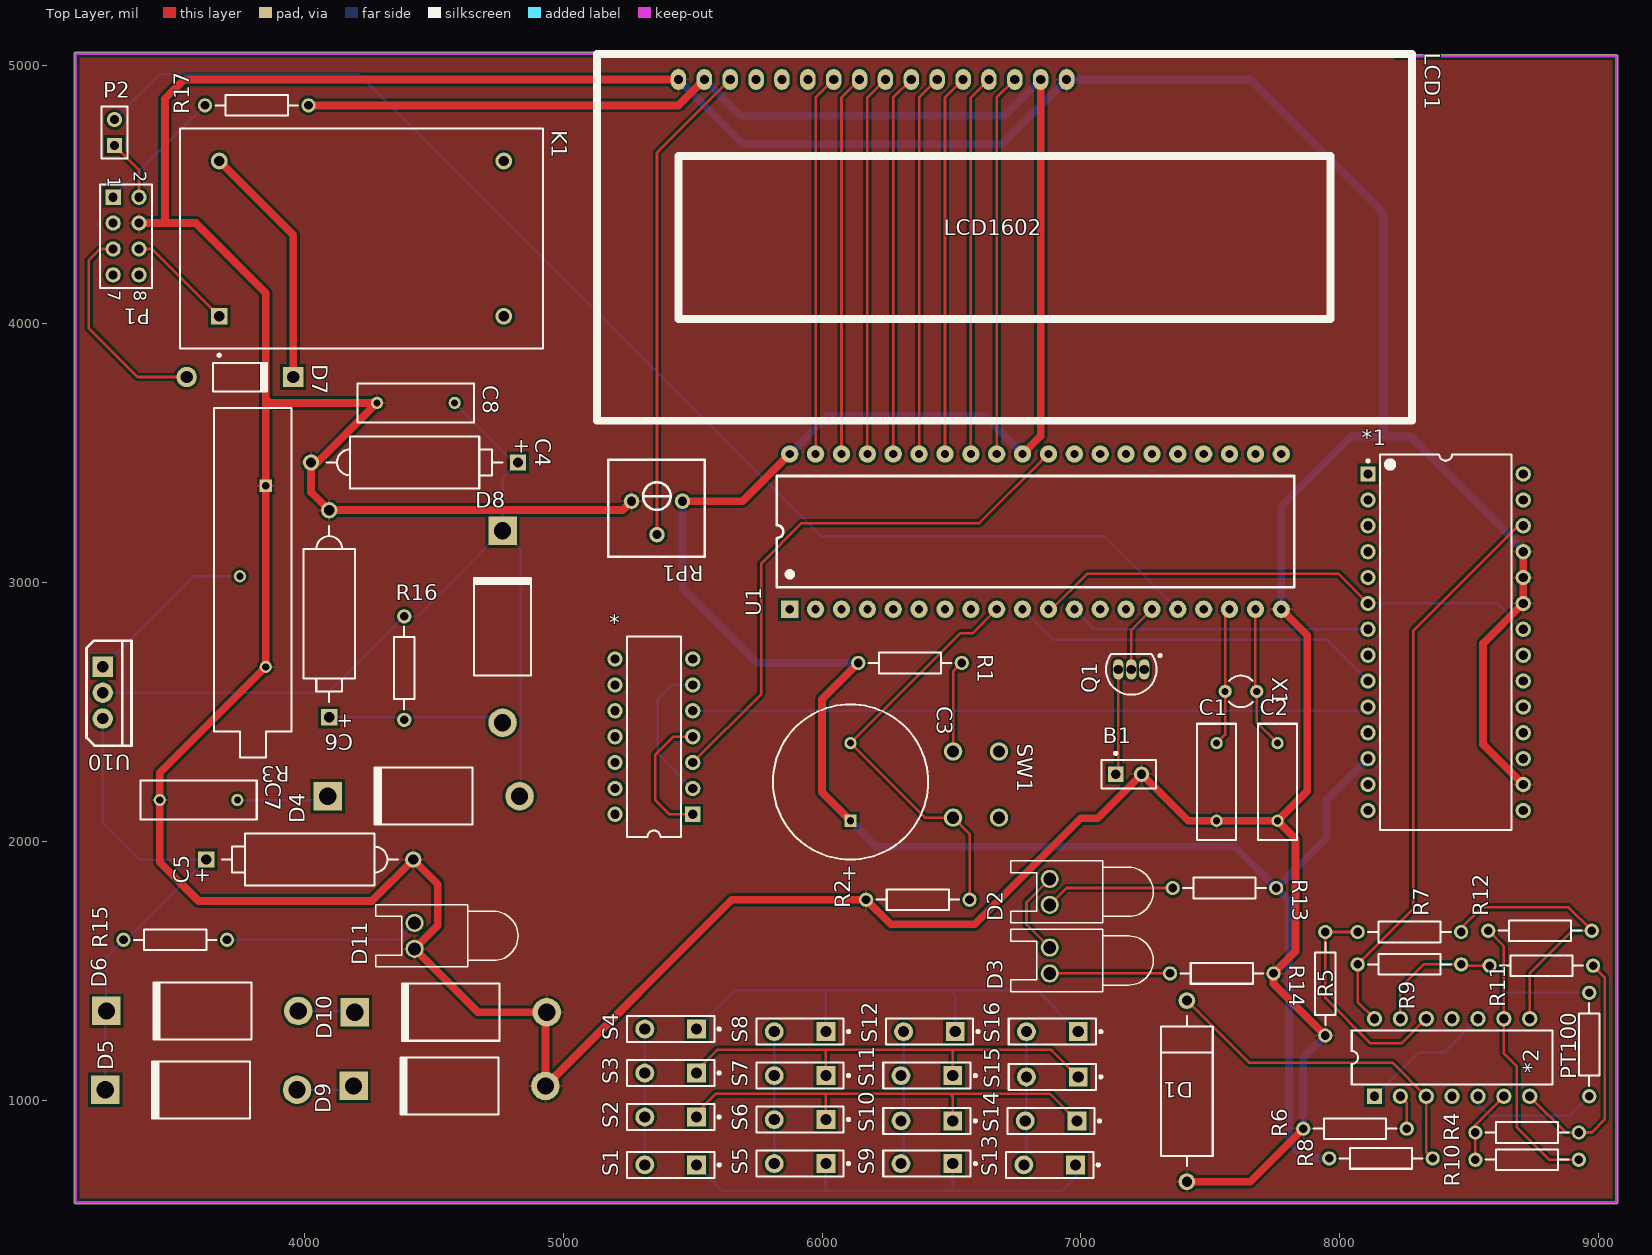
[diagram p0: Top Layer view]
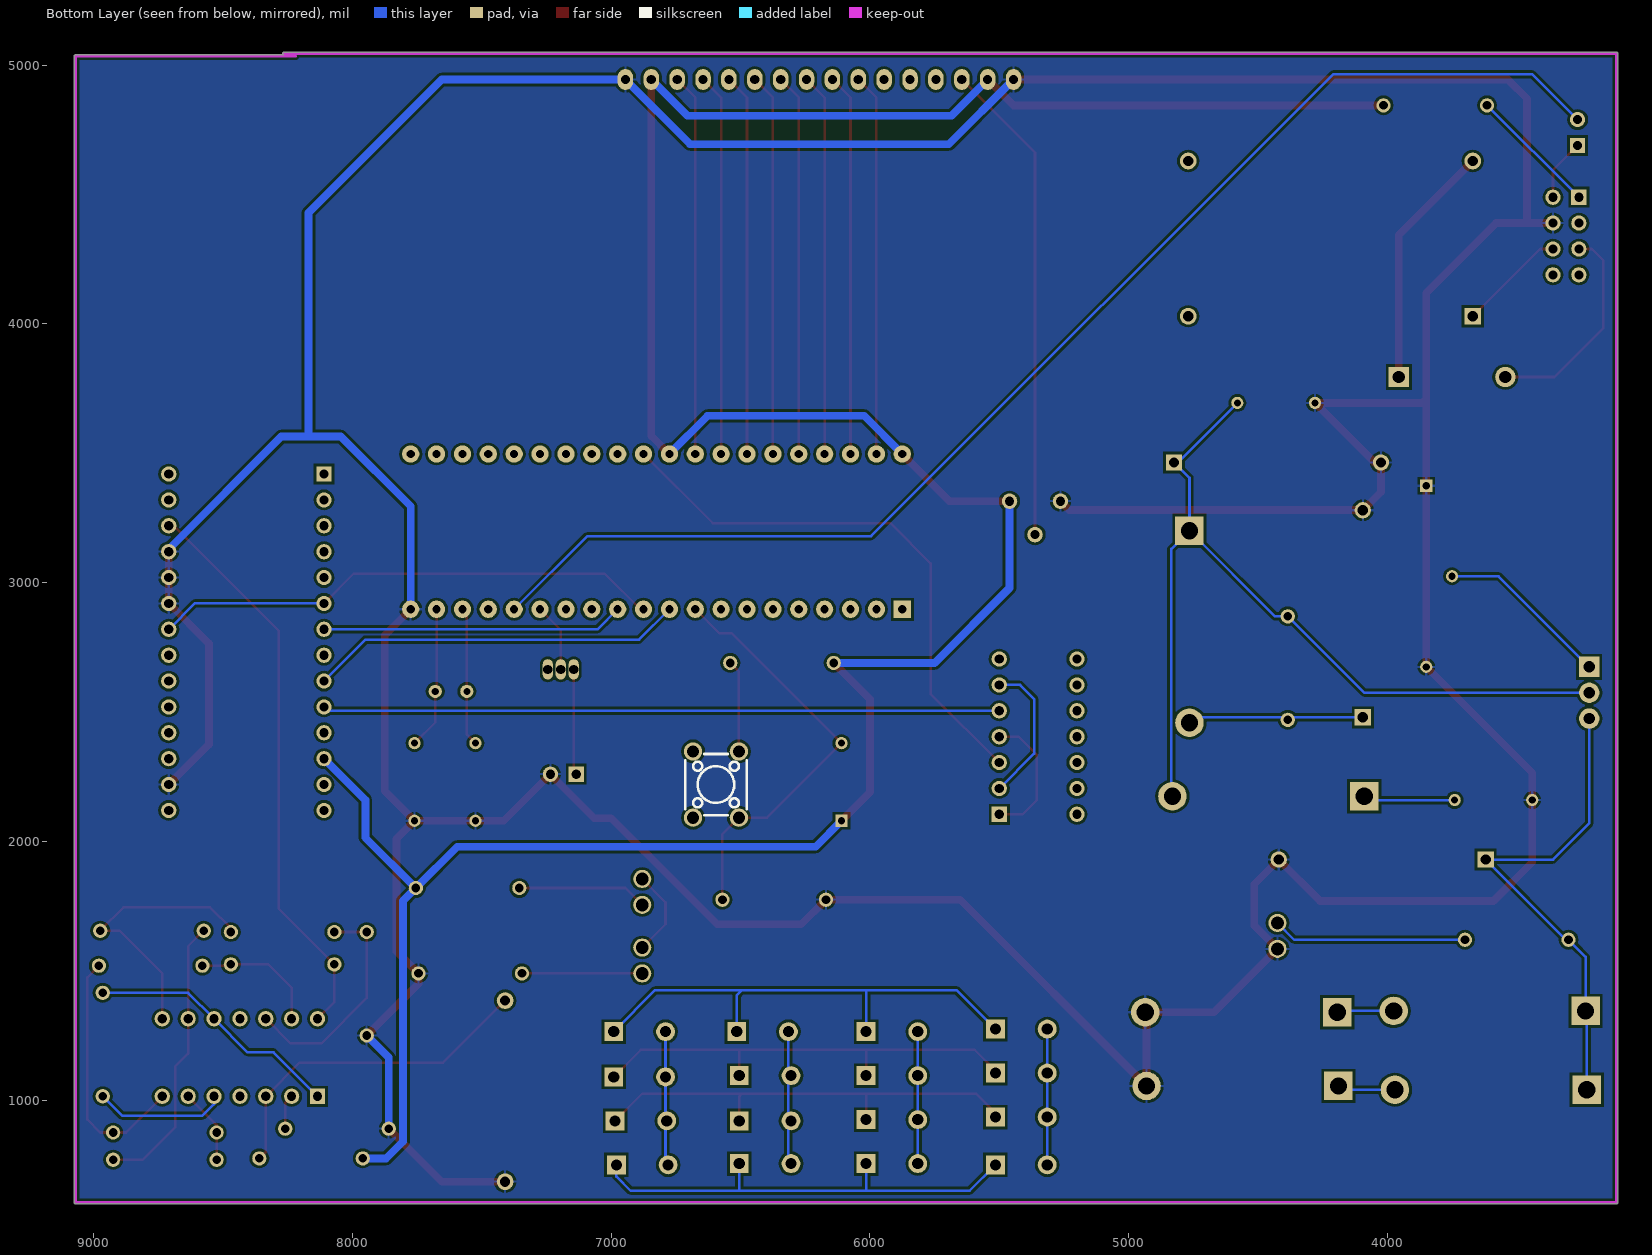
[diagram p1: Bottom Layer view, seen from below]
# Altium PCB MISC80626.PcbDoc
Units mil, origin at the board's own origin, x right, y up, seen from the top; angles counter-clockwise.
Board outline 5965.03 x 4450.03 mil, 2 copper layers (Top Layer, Bottom Layer); 67 components, 63 nets, 250 pads, 0 vias.

## Layer stack, top to bottom (the 12.6 mil dielectric is the usual default, probably not edited)
Top Solder: solder mask 0.4, Solder Resist, Dk 3.5
Top Layer: signal copper 1.4
Dielectric 1: dielectric 12.6, FR-4, Dk 4.8
Bottom Layer: signal copper 1.4
Bottom Solder: solder mask 0.4, Solder Resist, Dk 3.5

## Board outline
3109.99,605 ccw(c3115,605) 3115,599.99 9070,599.99 ccw(c9070,605) 9075.01,605 9075.01,5035 ccw(c9070,5035) 9070,5040.02 8265.55,5040.02 ccw(c8265,5045) 8270.01,5045 ccw(c8265,5045) 8265,5050.02 3115,5050.02 ccw(c3115,5045) 3109.99,5045

## Design rules (kind name [scope] priority, off if disabled: settings)
Clearance [All] p1: gap=10 ignorepadtopadclearanceinfootprint=FALSE except(0: Arc-Hole Track-Hole SMDPad-Hole THPad-Hole Via-Hole Fill-Hole Poly-Hole Region-Hole Text-Hole)
MinimumSolderMaskSliver [All] p1: minsoldermaskwidth=0
PolygonConnect [All] p1: connectstyle=Relief reliefconductorwidth=10 reliefentries=4 polygonreliefangle="90 Angle" airgapwidth=10
RoutingVias [All] p1: holewidth=28 width=50 viastyle="Through Hole" minholewidth=28 minwidth=50 maxholewidth=28 maxwidth=50
SilkToSilkClearance [All] p1: silktosilkclearance=0
SilkToSolderMaskClearance [IsPad] p1: minsilkscreentomaskgap=0 clearancetoexposedcopper=TRUE
SolderMaskExpansion [All] p1: expansion=4
Width [All] p1: maxlimit=30 minlimit=10 preferedwidth=10
27 further rules are at their usual default settings.

## Components (designator, comment, footprint, x,y, rotation, side; value= is the part's Value field where it differs from the comment)
* "74LS74" 646-06 5350,2405 r90 top
*1 "ADC0809" N28B 8410,2770 r0 top
*2 "LM324N" 646-06 8435,1165 r0 top
B1 "DC5V" PIN2 7135,2260 r0 top
C1 "104" RAD-0.3 7525,2230 r90 top
C2 "104" RAD-0.3 7760,2230 r90 top
C3 "10UF/16V" RB7.6-15 6110,2230 r270 top
C4 "Cap Pol2" POLAR0.8 4425,3465 r0 top
C5 "Cap Pol2" POLAR0.8 4020,1930 r180 top
C6 "Cap Pol2" POLAR0.8 4095,2880 r270 top
C7 "104" RAD-0.3 3590,2160 r0 top
C8 "104" RAD-0.3 4430,3695 r0 top
D1 "1N4733A" DIODE-0.7 7410,1035 r90 top
D2 "LED0" LED-0 6880,1805 r90 top
D3 "LED0" LED-0 6880,1540 r90 top
D4 "DIODE" DO-201AD 4460,2175 r180 top
D5 "DIODE" DO-201AD 3600,1040 r180 top
D6 "DIODE" DO-201AD 3605,1345 r180 top
D7 "Diode 1N4007" DO-41 3750,3795 r0 top
D8 "DIODE" DO-201AD 4765,2830 r90 top
D9 "DIODE" DO-201AD 4560,1055 r180 top
D10 "DIODE" DO-201AD 4565,1340 r180 top
D11 "LED0" LED-0 4425,1635 r90 top
K1 "Relay-SPST" MODULE4 4220,4330 r0 top
LCD1 "LCD 1602" LCD1602 5445,4945 r0 top
P1 "4N27" HDR2X4 3260,4490 r270 top
P2 "74F04" HDR1X2 3265,4690 r90 top
PT100 "30K" AXIAL-0.4 8965,1215 r270 top
Q1 "2N3906" TO-92A 7195,2665 r90 top
R1 "10K" AXIAL-0.4 6340,2690 r0 top
R2 "10K" AXIAL-0.4 6370,1775 r180 top
R3 "Res Tap" VR3 3800,3025 r270 top
R4 "450" AXIAL-0.4 8725,875 r180 top
R5 "1K" AXIAL-0.4 7945,1450 r90 top
R6 "3.3K" AXIAL-0.4 8060,890 r180 top
R7 "1K" AXIAL-0.4 8270,1650 r0 top
R8 "1K" AXIAL-0.4 8160,775 r180 top
R9 "1K" AXIAL-0.4 8270,1525 r0 top
R10 "30K" AXIAL-0.4 8725,770 r0 top
R11 "1K" AXIAL-0.4 8780,1520 r180 top
R12 "450" AXIAL-0.4 8775,1655 r180 top
R13 "250" AXIAL-0.4 7555,1820 r0 top
R14 "250" AXIAL-0.4 7545,1490 r0 top
R15 "30K" AXIAL-0.4 3500,1620 r180 top
R16 "200" AXIAL-0.4 4385,2670 r90 top
R17 "500" AXIAL-0.4 3815,4845 r180 top
RP1 "10K" 电位器 5360,3300 r180 top
S1 "SW-PB" SPST-2 5415,750 r180 top
S2 "SW-PB" SPST-2 5415,935 r180 top
S3 "SW-PB" SPST-2 5415,1105 r180 top
S4 "SW-PB" SPST-2 5415,1275 r180 top
S5 "SW-PB" SPST-2 5915,755 r180 top
S6 "SW-PB" SPST-2 5915,925 r180 top
S7 "SW-PB" SPST-2 5915,1095 r180 top
S8 "SW-PB" SPST-2 5915,1265 r180 top
S9 "SW-PB" SPST-2 6405,755 r180 top
S10 "SW-PB" SPST-2 6405,920 r180 top
S11 "SW-PB" SPST-2 6405,1095 r180 top
S12 "SW-PB" SPST-2 6415,1265 r180 top
S13 "SW-PB" SPST-2 6880,750 r180 top
S14 "SW-PB" SPST-2 6885,920 r180 top
S15 "SW-PB" SPST-2 6890,1090 r180 top
S16 "SW-PB" SPST-2 6890,1265 r180 top
SW1 "6x6x5" 四脚轻触开关 6595,2220 r270 top
U1 "STC89C5xx" DIP40 6825,3197.46 r90 top
U10 "LM317" TO220A 3220,2575 r270 top
X1 "12MHz" R38 7618.98,2580 r270 top

## Footprints (in the part's own frame and the unit in brackets; to place one, negate y for a bottom-side part, rotate by r counter-clockwise, add the part's x,y. Pads: shape width x height; smd on the part's side, far side on the other; paste and mask are expansions set on the pad)
646-06 [mm] "DIP; 14 Leads; Row Spacing 7.62 mm; Pitch 2.54 mm"
  rect 1.5x1.5 hole 0.9: 1(-7.62,-3.81)
  round 1.5 hole 0.9: 2(-5.08,-3.81) 3(-2.54,-3.81) 4(0,-3.81) 5(2.54,-3.81) 6(5.08,-3.81) 7(7.62,-3.81) 8(7.62,3.81) 9(5.08,3.81) 10(2.54,3.81) 11(0,3.81) 12(-2.54,3.81) 13(-5.08,3.81) 14(-7.62,3.81)
  silkscreen extent -9.85,-2.65 9.85,2.65
AXIAL-0.4 [mm] "Axial Device, Thru-Hole; 2 Leads; 0.4 in Pin Spacing"
  round 1.4 hole 0.85: 1(-5.08,0) 2(5.08,0)
  silkscreen extent -4.06,-1.02 4.06,1.02
DIODE-0.7 [mm] "Diode, Thru-Hole; 2 Leads; 0.7 in Pin Spacing"
  round 1.65 hole 1: 1(-8.89,0) 2(8.89,0)
  silkscreen extent -7.37,-2.54 7.37,2.54
DIP40 [mm]
  rect 1.7x1.7 hole 0.8: 1(-7.62,24.13)
  round 1.7 hole 0.8: 2(-7.62,21.59) 3(-7.62,19.05) 4(-7.62,16.51) 5(-7.62,13.97) 6(-7.62,11.43) 7(-7.62,8.89) 8(-7.62,6.35) 9(-7.62,3.81) 10(-7.62,1.27) 11(-7.62,-1.27) 12(-7.62,-3.81) 13(-7.62,-6.35) 14(-7.62,-8.89) 15(-7.62,-11.43) 16(-7.62,-13.97) 17(-7.62,-16.51) 18(-7.62,-19.05) 19(-7.62,-21.59) 20(-7.62,-24.13) 21(7.62,-24.13) 22(7.62,-21.59) 23(7.62,-19.05) 24(7.62,-16.51) 25(7.62,-13.97) 26(7.62,-11.43) 27(7.62,-8.89) 28(7.62,-6.35) 29(7.62,-3.81) 30(7.62,-1.27) 31(7.62,1.27) 32(7.62,3.81) 33(7.62,6.35) 34(7.62,8.89) 35(7.62,11.43) 36(7.62,13.97) 37(7.62,16.51) 38(7.62,19.05) 39(7.62,21.59) 40(7.62,24.13)
  silkscreen extent -5.46,-25.4 5.46,25.4, body extent -7.91,-26.19 7.65,26.16, height 4.7
DO-41 [mm] "Diode, Axial; Body 5.2 x 2.7 mm (LxDia. max), Lead Dia. 0.86 mm (max)"
  round 2 hole 1.2: 1(-5.23,0)
  rect 2x2 hole 1.2: 2(5.23,0)
  silkscreen extent -2.65,-1.4 2.75,1.4
DO-201AD [mm] "Diode, Axial; Body 9.5 x 5.6 mm (LxDia. max), Lead Dia. 1.32 mm (max)"
  round 2.8 hole 1.7: 1(-9.42,0)
  rect 2.8x2.8 hole 1.7: 2(9.42,0)
  silkscreen extent -4.8,-2.8 4.9,2.8
HDR1X2 [mm] "Connector; Header; 2 Position"
  rect 1.5x1.5 hole 0.9: 1(0,0)
  round 1.5 hole 0.9: 2(2.54,0)
  silkscreen extent -1.27,-1.27 3.81,1.27
HDR2X4 [mm] "Connector; Header; 4x2 Position"
  rect 1.5x1.5 hole 0.9: 1(0,0)
  round 1.5 hole 0.9: 2(0,2.54) 3(2.54,0) 4(2.54,2.54) 5(5.08,0) 6(5.08,2.54) 7(7.62,0) 8(7.62,2.54)
  silkscreen extent -1.27,-1.27 8.89,3.81
LCD1602 [mil]
  oval 60x80 hole 35.43: 1(0,0) 2(100,0) 3(200,0) 4(300,0) 5(400,0) 6(500,0) 7(600,0) 8(700,0) 9(800,0) 10(900,0) 11(1000,0) 12(1100,0) 13(1200,0) 14(1300,0) 15(1400,0) 16(1500,0)
  silkscreen extent -315,-1319 2835,98, body extent -315,-1357 2854,80, height 414
LED-0 [mil] "LED; 2 Leads"
  round 70 hole 50: 1(50,0) 2(-50,0)
  silkscreen extent -120,-400 120,150
MODULE4 [mm] "DIP; 4 Round Pins; Row Space 27.94 mm; Pitch 15.24 mm"
  rect 1.65x1.65 hole 1: 1(-13.97,-7.62)
  round 1.65 hole 1: 2(-13.97,7.62) 3(13.97,-7.62) 4(13.97,7.62)
  silkscreen extent -17.8,-11.57 17.8,10.8, body extent -17.8,-10.8 17.8,10.8, height 14
N28B [mm] "DIP, 28-Leads, Row Spacing 15.24mm, Pitch 2.54mm, Body 35.73x12.95mm"
  rect 1.5x1.5 hole 0.9: 1(-7.62,16.51)
  round 1.5 hole 0.9: 2(-7.62,13.97) 3(-7.62,11.43) 4(-7.62,8.89) 5(-7.62,6.35) 6(-7.62,3.81) 7(-7.62,1.27) 8(-7.62,-1.27) 9(-7.62,-3.81) 10(-7.62,-6.35) 11(-7.62,-8.89) 12(-7.62,-11.43) 13(-7.62,-13.97) 14(-7.62,-16.51) 15(7.62,-16.51) 16(7.62,-13.97) 17(7.62,-11.43) 18(7.62,-8.89) 19(7.62,-6.35) 20(7.62,-3.81) 21(7.62,-1.27) 22(7.62,1.27) 23(7.62,3.81) 24(7.62,6.35) 25(7.62,8.89) 26(7.62,11.43) 27(7.62,13.97) 28(7.62,16.51)
  silkscreen extent -7.74,-18.45 6.45,18.45, body extent -7.42,-18.42 7.42,18.42, height 5.34
PIN2 [mm] "Photosensitive Diode; 2 Leads"
  rect 1.5x1.5 hole 0.9: 1(0,0)
  round 1.5 hole 0.9: 2(2.54,0)
  silkscreen extent -1.4,-1.4 3.94,2.17
POLAR0.8 [mm] "Polarized Capacitor; 2 Leads"
  rect 1.6x1.6 hole 1: 1(10.16,0)
  round 1.6 hole 1: 2(-10.16,0)
  silkscreen extent -8.64,-2.54 8.64,2.54
R38 [mm] "Crystal, Thru-Hole; 2 Leads; Body 3.1 x 8.2 mm (Dia.xH)"
  round 1.3 hole 0.7: 1(0,1.55) 2(0,-1.55)
  silkscreen extent -1.55,-1.19 1.55,1.17
RAD-0.3 [mm] "Radial Cap, Thru-Hole; 2 Leads; 0.3 in Pin Spacing"
  round 1.2 hole 0.7: 1(-3.81,0) 2(3.81,0)
  silkscreen extent -5.71,-1.91 5.71,1.91
RB7.6-15 [mm] "Polarized Capacitor (Radial); 2 Leads"
  rect 1.2x1.2 hole 0.7: 1(3.81,0)
  round 1.2 hole 0.7: 2(-3.81,0)
  silkscreen extent -7.62,-7.62 7.62,7.62
SPST-2 [mm] "Switch; 2 Leads"
  rect 1.85x1.85 hole 1.1: 1(-2.54,0)
  round 1.85 hole 1.1: 2(2.54,0)
  silkscreen extent -4.89,-1.27 4.28,1.27
TO220A [mm] "220，3脚晶体管"
  rect 2x2 hole 1.1: 1(-2.54,0)
  round 2 hole 1.1: 2(0,0) 3(2.54,0)
  silkscreen extent -5.08,-1.6 5.21,2.82, body extent -5.08,-1.45 5.22,2.98, height 18.5
TO-92A [mm] "TO, Flat Index; 3 In-Line, Axial Leads; Body Dia. 4.5mm; Leads 0.51 x 0.48 mm (max)"
  oval 2x1 hole 0.9: 1(0,-1.27) 2(0,0) 3(0,1.27)
  silkscreen extent -2.48,-2.96 1.5,2.48, body extent -2.48,-2.5 1.5,2.5, height 6.86
VR3 [mm] "Thru-Hole; 3 Leads"
  rect 1.2x1.2 hole 0.7: 1(-8.89,1.27)
  round 1.2 hole 0.7: 2(0,-1.27) 3(8.89,1.27)
  silkscreen extent -16.51,-3.81 17.78,3.81
四脚轻触开关 [mm]
  round 1.8 hole 1.2 paste+0 mask+0.102: 1(3.25,2.25) 2(-3.25,2.25) 3(3.25,-2.25) 4(-3.25,-2.25)
电位器 [mil]
  round 60 hole 35.43 paste+0 mask+2: 1(96.41,-15.12) 2(-2.02,114.1) 3(-100.44,-15.12)
  silkscreen extent -187,-175 187,199

## Part data
* *1 *2: library part Component_1
B1: library part BEEP, "Buzzer"
C1 C2 C7 C8: library part C-CC, "Through-hole ceramic capacitor"
C3: library part C-CAP, "Through-hole electrolytic capacitor"
C4 C5 C6: "Polarized Capacitor (Axial)"
D1: library part "D Zener", "Zener Diode"
D2 D3 D11: "Typical INFRARED GaAs LED"
D4 D5 D6 D7 D8 D9 D10: library part "Diode 1N5400", "3 Amp General Purpose Rectifier"
K1: "Single-Pole Single-Throw Relay"
P1: library part "Header 4X2A", "Header, 4-Pin, Dual row"
P2: library part "Header 2", "Header, 2-Pin"
PT100 R1 R2 R4 R5 R6 R7 R8 R9 R10 R11 R12 R13 R14 R15 R16 R17: library part R-CRR, "Through-hole colour-band resistor"
Q1: "PNP General Purpose Amplifier"
R3: "Tapped Resistor"
RP1: library part RP-ID, "Plug-in single-gang potentiometer"
S1 S2 S3 S4 S5 S6 S7 S8 S9 S10 S11 S12 S13 S14 S15 S16: "Switch"
SW1: library part "TSW DIP-6x6", "Through-hole 6x6 tactile switch"
U1: "STC microcontroller"
U10: "Adjustable linear regulator IC"
X1: library part XTAL-2, "2-pin crystal oscillator"

## Nets (pads, with @x,y where several pads share a name; then routed paths per layer and width w, separated by ;. In a path a pad name is that pad's centre, name@x,y a point inside that pad or via, vN(x,y) a via of type N, cw(c..) or ccw(c..) an arc to the next point about the centre after c; other vN are vias at no path point)
+12V: D7.2 K1.2 | length 953.4
  Top Layer w30: K1.2 3955.91,4344.09 D7.2
ALE: *.3 U1.30 | length 2164.8
  Top Layer w10: *.3 5765,2570 5765,3075 5920,3230 6607.54,3230 U1.30
CLOCK: *1.10 *.5 | length 2616.2
  Bottom Layer w10: *.5 8095,2505 *1.10
EN: *1.9 U1.10 | length 1449.9
  Bottom Layer w10: U1.10 6892.46,2780 7950,2780 *1.9
EOC: *1.7 U1.12 | length 1167.1
  Bottom Layer w10: U1.12 7052.46,2820 *1.7
GND: *1.16 *1.23 *1.24 *1.25 B1.2 C1.1 C2.1 C4.2 C5.2 C6.2 C7.1 C8.1 D1.1 D9.1 D10.1 D11.2 LCD1.1 LCD1.16 P1.4 R2.2 R3.1 R3.3 R5.1 R6.2 R14.2 RP1.1 U1.20 | length 23050
  Top Layer w30: P1.4 3460,4390 ; RP1.1 5229.46,3280.98 4095,3280.98 C6.2 4025,3350 C4.2 4050,3465 C8.1 3865,3695 3850,3710 ; LCD1.1 3535,4945 3460,4870 3460,4390 ; D1.1 7655,685 R6.2 ; U1.20 7875,2797.46 7875,2195 C2.1 ; R5.1 7745,1450 R14.2 7830,1575 7830,2010 C2.1 ; *1.16 8555,2375 8555,2765 *1.23 *1.24 *1.25 ; 3460,4390 3580,4390 3850,4120 3850,3710 ; 3850,3710 R3.1 R3.3 3440,2265 C7.1 3440,1920 3590,1770 4260,1770 C5.2 4515,1835 4515,1675 D11.2 4670,1340 D10.1 4930.87,1335 D9.1 5650.87,1775 R2.2 6265,1680 6590,1680 7000,2090 7065,2090 B1.2 7415,2080 C1.1 C2.1
  Bottom Layer w30: LCD1.1 5695,4695 6695,4695 LCD1.16 7655,4945 8170,4430 8170,3565 ; U1.20 7775,3295 8045,3565 8170,3565 ; R6.2 7860,1165 R5.1 ; *1.25 8710,3130 8275,3565 8170,3565
LCD_EN: U1.14
LCD_RS: U1.13
LEC: U1.17
LED: D2.1 D3.1 | length 339.6
  Top Layer w10: D3.1 6790,1680 6790,1765 D2.1
Net*1_26: *1.26 *2.14 R9.1 | length 2208.7
  Top Layer w10: *2.14 8070,1380 R9.1 8285,1740 8285,2815 8690,3220 *1.26
Net*2_1: *2.1 *2.10 PT100.1 | length 995.7
  Bottom Layer w10: *2.1 8305,1185 8405,1185 *2.10 8635,1415 PT100.1
Net*2_2: *2.2 R6.1 | length 135.4
  Top Layer w10: *2.2 8260,990 R6.1
Net*2_3: *2.3 D1.2 R8.1 | length 1328.6
  Top Layer w10: D1.2 7650,1145 8205,1145 *2.3 8335,800 R8.1
Net*2_5: *2.5 PT100.2 | length 509.7
  Bottom Layer w10: *2.5 8535,985 8580,940 8890,940 PT100.2
Net*2_6: *2.6 R4.2 R10.1 | length 290.6
  Top Layer w10: R10.1 R4.2 8525,905 *2.6
Net*2_7: *2.7 R4.1 R11.1 | length 982.3
  Top Layer w10: *2.7 8875,875 R4.1 8975,875 9025,925 9025,1475 R11.1
Net*2_8: *2.8 R7.2 R12.1 | length 1073.8
  Top Layer w10: R7.2 8470,1665 8550,1745 8885,1745 R12.1 8900,1655 8735,1490 *2.8
Net*2_9: *2.9 R10.2 R12.2 | length 1097.3
  Top Layer w10: R12.2 8635,1595 *2.9 8635,1180 8685,1130 8685,895 8810,770 R10.2
Net*2_12: *2.12 R5.2 R7.1 | length 881.8
  Top Layer w10: R7.1 R5.2 7945,1395 8120,1220 8240,1220 *2.12
Net*2_13: *2.13 R9.2 R11.2 | length 504.4
  Top Layer w10: *2.13 8235,1435 8325,1525 R9.2 8475,1520 R11.2
Net*_1: *.1 *.4 | length 516.8
  Top Layer w10: *.1 5410,2105 5355,2160 5355,2335 5425,2405 *.4
Net*_2: *.2 *.6 | length 558.7
  Bottom Layer w10: *.2 5365,2340 5365,2550 5420,2605 *.6
NetB1_1: B1.1 Q1.3 | length 409.1
  Top Layer w10: B1.1 7145,2270 Q1.3
NetC1_2: C1.2 U1.18 X1.2 | length 538.2
  Top Layer w10: C1.2 7557.95,2412.95 X1.2 7557.95,2880.42 U1.18
NetC2_2: C2.2 U1.19 X1.1 | length 552.7
  Top Layer w10: U1.19 7675,2585 X1.1 7680,2460 C2.2
NetC3_2: C3.2 R2.1 SW1.3 U1.9 | length 1638.4
  Top Layer w10: R2.1 6570,2028.46 SW1.3 6397.95,2092.05 C3.2 6535,2805 6582.54,2805 U1.9
NetC4_1: C4.1 C8.2 D4.1 D8.2 R16.2 U10.2 | length 3490.2
  Bottom Layer w10: U10.2 4090,2575 R16.2 4434.13,2870 D8.2 ; C8.2 4810,3465 C4.1 4765,3405 D8.2 ; D4.1 4835.12,2179.25 4835.12,3130.75 D8.2
NetC5_1: C5.1 D5.2 D6.2 R15.2 U10.3 | length 1920.7
  Bottom Layer w10: U10.3 3220,2070 3360,1930 C5.1 3310,1620 R15.2 3234.13,1554.13 D6.2 3229.13,1340 D5.2
NetC6_1: C6.1 D8.1 R16.1 | length 678.6
  Bottom Layer w10: C6.1 4744.13,2480 D8.1
NetC7_2: C7.2 D4.2 | length 355.3
  Bottom Layer w10: C7.2 4074.13,2160 D4.2
NetD2_2: D2.2 R13.1 | length 501.9
  Top Layer w10: D2.2 6945,1820 R13.1
NetD3_2: D3.2 R14.1 | length 465
  Top Layer w10: D3.2 R14.1
NetD5_1: D5.1 D9.2 | length 224.5
  Bottom Layer w10: D5.1 4174.13,1040 D9.2
NetD6_1: D6.1 D10.2 | length 220.3
  Bottom Layer w10: D6.1 4189.13,1345 D10.2
NetD7_1: D7.1 P1.5 | length 831.4
  Top Layer w10: P1.5 3210,4290 3165,4245 3165,3985 3355,3795 D7.1
NetD11_1: D11.1 R15.1 | length 751.9
  Bottom Layer w10: R15.1 4360,1620 D11.1
NetK1_1: K1.1 P1.6 | length 417.7
  Top Layer w10: P1.6 3410,4290 K1.1
NetLCD1_3: LCD1.3 RP1.2 | length 1876.3
  Top Layer w10: RP1.2 5362.02,4662.02 LCD1.3
NetLCD1_7: LCD1.7 U1.39 | length 1476.5
  Top Layer w10: U1.39 5975,4875 LCD1.7
NetLCD1_8: LCD1.8 U1.38 | length 1476.5
  Top Layer w10: U1.38 6075,4875 LCD1.8
NetLCD1_9: LCD1.9 U1.37 | length 1476.5
  Top Layer w10: U1.37 6175,4875 LCD1.9
NetLCD1_10: LCD1.10 U1.36 | length 1476.5
  Top Layer w10: U1.36 6275,4875 LCD1.10
NetLCD1_11: LCD1.11 U1.35 | length 1476.5
  Top Layer w10: U1.35 6375,4875 LCD1.11
NetLCD1_12: LCD1.12 U1.34 | length 1476.5
  Top Layer w10: U1.34 6475,4875 LCD1.12
NetLCD1_13: LCD1.13 U1.33 | length 1476.5
  Top Layer w10: U1.33 6575,4875 LCD1.13
NetLCD1_14: LCD1.14 U1.32 | length 1476.5
  Top Layer w10: U1.32 6675,4875 LCD1.14
NetP1_1: P1.1 R17.2 | length 502
  Bottom Layer w10: P1.1 R17.2
NetP1_2: P1.2 P2.1 | length 239.4
  Top Layer w10: P2.1 3360,4595 P1.2
NetR1_2: R1.2 SW1.4 | length 356
  Top Layer w10: SW1.4 6506.42,2656.42 R1.2
NetR3_2: R3.2 U10.1 | length 675
  Bottom Layer w10: U10.1 3570,3025 R3.2
NetS1_1: S1.1 S5.1 S9.1 S13.1 | length 1786.3
  Bottom Layer w10: S1.1 5615,650 6010,650 ; S5.1 6015,655 6010,650 ; S9.1 6505,650 ; S13.1 6980,705 6925,650 6505,650 ; 6010,650 6505,650
NetS1_2: S1.2 S2.2 S3.2 S4.2 | length 525
  Bottom Layer w10: S1.2 S2.2 S3.2 S4.2
NetS2_1: S2.1 S6.1 S10.1 S14.1 | length 1768.7
  Top Layer w10: S2.1 5515,950 5590,1025 6015,1025 ; S6.1 6015,1025 ; S10.1 6505,1015 6495,1025 ; S14.1 6880,1025 6495,1025 ; 6015,1025 6495,1025
NetS3_1: S3.1 S7.1 S11.1 S15.1 | length 1761.6
  Top Layer w10: S3.1 5515,1115 5595,1195 6015,1195 ; S7.1 6015,1195 ; S11.1 6505,1195 ; S15.1 6885,1195 6505,1195 ; 6015,1195 6505,1195
NetS4_1: S4.1 S8.1 S12.1 S16.1 | length 1931.7
  Bottom Layer w10: S4.1 5665,1425 6015,1425 ; S8.1 6015,1425 ; S12.1 6515,1405 6495,1425 ; S16.1 6830,1425 6495,1425 ; 6015,1425 6495,1425
NetS5_2: S5.2 S6.2 S7.2 S8.2 | length 510
  Bottom Layer w10: S5.2 S6.2 S7.2 S8.2
NetS9_2: S9.2 S10.2 S11.2 S12.2 | length 514.1
  Bottom Layer w10: S9.2 6315,765 S12.2
NetS13_2: S13.2 S14.2 S15.2 S16.2 | length 519.1
  Bottom Layer w10: S13.2 6790,760 S15.2 S16.2
P1.4: Q1.2 U1.15 | length 265.6
  Top Layer w10: Q1.2 7195,2817.46 U1.15
START: *1.6 *1.22 U1.11 | length 1981
  Top Layer w10: U1.11 6887.46,2897.46 7025,3035 7995,3035 *1.6
  Bottom Layer w10: *1.6 8610,2920 *1.22
SWITCH: P2.2 U1.16 | length 5038.9
  Bottom Layer w10: P2.2 3440,4965 4210,4965 5995,3180 7092.46,3180 U1.16
VCC: *1.12 C3.1 LCD1.2 LCD1.15 R1.1 R8.2 R13.2 R17.1 RP1.3 U1.31 U1.40 | length 11407.2
  Top Layer w30: R17.1 5445,4845 LCD1.2 ; RP1.3 5692.65,3315.12 U1.40 ; C3.1 6000,2190 6000,2550 R1.1 ; U1.31 6845,3567.46 LCD1.15
  Bottom Layer w30: RP1.3 5460.44,2979.56 5750,2690 R1.1 ; LCD1.2 5685,4805 6705,4805 LCD1.15 ; U1.40 6022.54,3645 6627.46,3645 U1.31 ; C3.1 6210,1980 7595,1980 R13.2 ; R8.2 7870,775 7805,840 7805,1770 R13.2 ; *1.12 7950,2160 7950,2015 R13.2
pads on no net: *1.1 *1.2 *1.3 *1.4 *1.5 *1.8 *1.11 *1.13 *1.14 *1.15 *1.17 *1.18 *1.19 *1.20 *1.21 *1.27 *1.28 *2.4 *2.11 *.7 *.8 *.9 *.10 *.11 *.12 *.13 *.14 K1.3 K1.4 LCD1.4 LCD1.5 LCD1.6 P1.3 P1.7 P1.8 Q1.1 SW1.1 SW1.2 U1.1 U1.2 U1.3 U1.4 U1.5 U1.6 U1.7 U1.8 U1.21 U1.22 U1.23 U1.24 U1.25 U1.26 U1.27 U1.28 U1.29

## Polygon pours and split planes (outlines as drawn)
GND on Bottom Layer "Top Layer-No Net" (solid, remove dead copper, pour order 0): 2405,5450 2415,5460 10080,5460 10080,1045 9320,285 9140,465 2590,465
GND on Top Layer "Top Layer-No Net" (solid, remove dead copper, pour order 2): 2545,5470 9895,5470 10005,5580 9870,5445 9870,175 2740,175 2605,310

## Keep-outs
Keep-Out Layer:
  lines w10: 3115,730 3115,4875 3115,5045 8265,5045 ; 3115,740 3115,605 4060,605 9057.93,605 9070,605 9070,5035 8220,5035